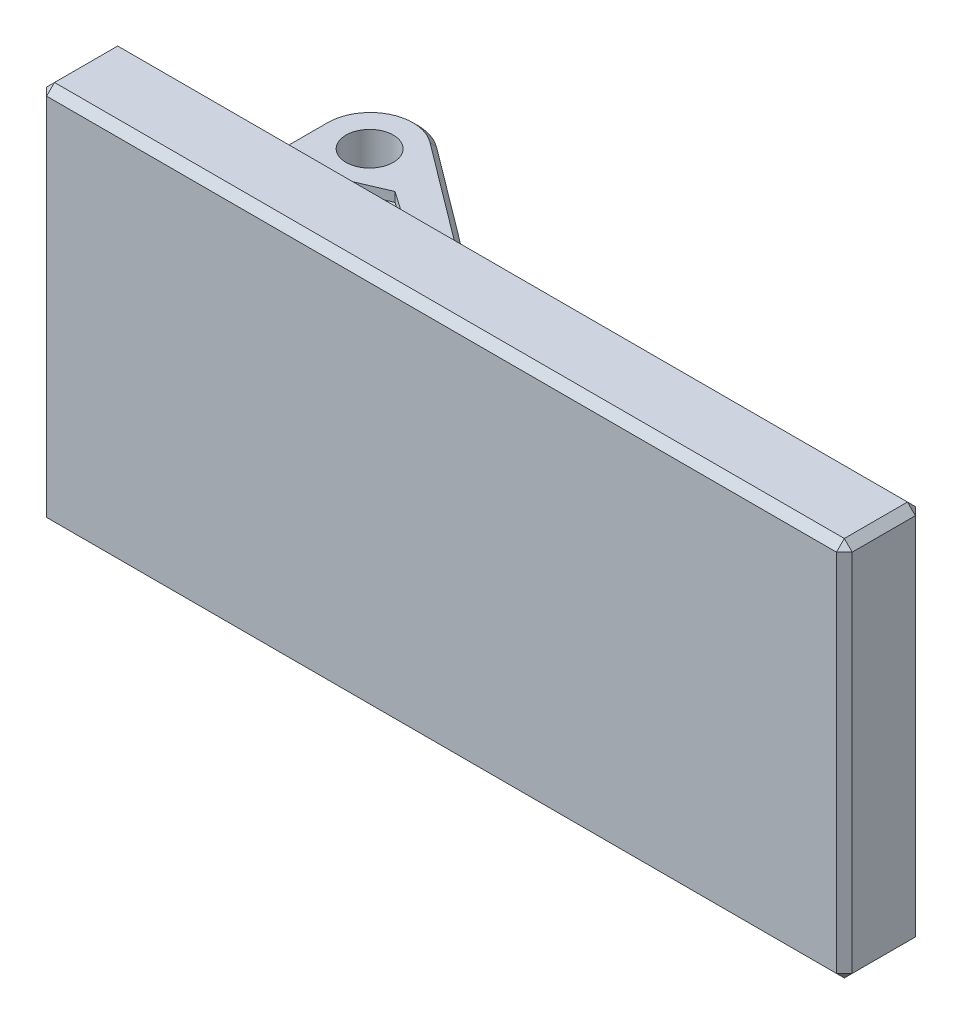
from build123d import *

# Parameters (mm, degrees)
SKETCH1_R               = 150
BOSS_EXTRUDE1_DEPTH     = 1000
FILLET2_R               = 300
SKETCH2_W               = 5102.2573033
SKETCH2_H               = 2410.803825692
BOSS_EXTRUDE2_DEPTH     = 500
SKETCH3_R               = 250
BOSS_EXTRUDE3_DEPTH     = 200
CUT_EXTRUDE1_DEPTH      = 750
CUT_EXTRUDE1_DEPTH_BACK = 150
SKETCH4_R               = 125
CHAMFER1_SIZE           = 30
CHAMFER2_SIZE           = 30
CUT_EXTRUDE3_DEPTH      = 60
CHAMFER3_SIZE           = 50
SKETCH7_W               = 1281.787678956
SKETCH7_H               = 560
CUT_EXTRUDE4_DEPTH      = 5144.935869353


with BuildPart() as part:
    # Sketch1 → Boss-Extrude1 (new body)
    with BuildSketch(Plane(origin=(0, 0, 0), x_dir=(1, 0, 0), z_dir=(0, 1, 0))):
        Polygon((0, 0), (0, -1500), (2000, -1500), align=None)
        with Locations(Location((306.027096019, -610.082997658, 0), (0, 0, 270))):
            Circle(SKETCH1_R, mode=Mode.SUBTRACT)
    extrude(amount=BOSS_EXTRUDE1_DEPTH)

    # Fillet2
    fillet2_edges = [part.edges().sort_by_distance(p)[0] for p in [
        (0, 500, 0),
    ]]
    fillet(fillet2_edges, radius=FILLET2_R)

    # Sketch2 → Boss-Extrude2 (add)
    with BuildSketch(Plane.XY.offset(1500)):
        with Locations((2151.177223521, 500)):
            Rectangle(SKETCH2_W, SKETCH2_H)
    extrude(amount=BOSS_EXTRUDE2_DEPTH)

    # Sketch3 → Boss-Extrude3 (add)
    with BuildSketch(Plane(origin=(0, 800, 0), x_dir=(1, 0, 0), z_dir=(0, 1, 0))):
        with Locations((2751.053965142, -1500)):
            Circle(SKETCH3_R)
    boss_extrude3 = extrude(amount=BOSS_EXTRUDE3_DEPTH)

    # Mirror1: Boss-Extrude3 across plane
    add(boss_extrude3.mirror(Plane.ZX.offset(500)))

    # Sketch4 → Cut-Extrude1 (cut, two sides: drawn at the far end of the back side and taken through both)
    with BuildSketch(Plane(origin=(0, 200, 0), x_dir=(1, 0, 0), z_dir=(0, 1, 0)).offset(-CUT_EXTRUDE1_DEPTH_BACK)):
        with Locations(Location((2751.053965142, -1500, 0), (0, 0, 270))):
            Circle(SKETCH4_R)
    extrude(amount=CUT_EXTRUDE1_DEPTH + CUT_EXTRUDE1_DEPTH_BACK, mode=Mode.SUBTRACT)

    # Chamfer1
    chamfer1_edges = [part.edges().sort_by_distance(p)[0] for p in [
        (2751.053965142, 1000, 1250),
        (2751.053965142, 0, 1250),
    ]]
    chamfer(chamfer1_edges, length=CHAMFER1_SIZE)

    # Chamfer2
    chamfer2_edges = [part.edges().sort_by_distance(p)[0] for p in [
        (0, 0, 1050),
        (0, 1000, 1050),
        (165.83592135, 0, 331.6718427),
        (165.83592135, 1000, 331.6718427),
        (1240, 0, 930),
        (1240, 1000, 930),
    ]]
    chamfer(chamfer2_edges, length=CHAMFER2_SIZE)

    # Sketch6 → Cut-Extrude3 (cut)
    with BuildSketch(Plane(origin=(0, 1000, 0), x_dir=(1, 0, 0), z_dir=(0, 1, 0))):
        Polygon((206.784286563, -1500), (206.784286563, -941.313978524), (621.042939875, -764.349116915), (1678.810180856, -1500), align=None)
    cut_extrude3 = extrude(amount=-CUT_EXTRUDE3_DEPTH, mode=Mode.SUBTRACT)

    # Mirror2: Cut-Extrude3 across plane
    add(cut_extrude3.mirror(Plane.ZX.offset(500)), mode=Mode.SUBTRACT)

    # Chamfer3
    chamfer3_edges = [part.edges().sort_by_distance(p)[0] for p in [
        (4702.305875171, 500, 1500),
        (4702.305875171, -705.401912846, 1750),
        (2151.177223521, 1705.401912846, 1500),
        (4702.305875171, 1705.401912846, 1750),
        (-399.951428129, 500, 1500),
        (-399.951428129, 1705.401912846, 1750),
        (2151.177223521, -705.401912846, 1500),
        (-399.951428129, -705.401912846, 1750),
        (4702.305875171, 500, 2000),
        (2151.177223521, 1705.401912846, 2000),
        (-399.951428129, 500, 2000),
        (2151.177223521, -705.401912846, 2000),
    ]]
    chamfer(chamfer3_edges, length=CHAMFER3_SIZE)

    # Sketch7 → Cut-Extrude4 (cut, through all)
    with BuildSketch(Plane(origin=(0, 0, 1500), x_dir=(-1, 0, 0), z_dir=(0, 0, -1))):
        with Locations((-1359.106160522, 500)):
            Rectangle(SKETCH7_W, SKETCH7_H)
    extrude(amount=CUT_EXTRUDE4_DEPTH, mode=Mode.SUBTRACT)


solid = part.part
